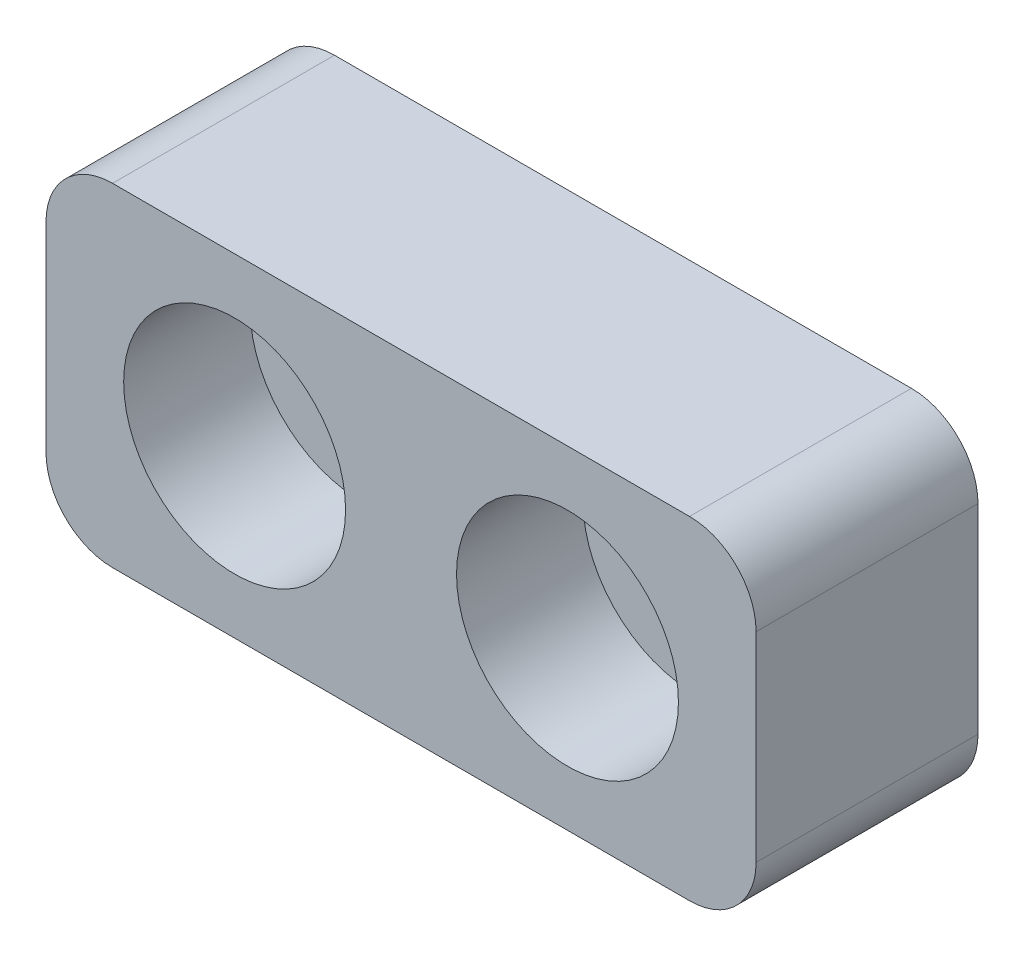
from build123d import *

# Parameters (mm, degrees)
SKETCH1_W                                            = 32
SKETCH1_H                                            = 15
BOSS_EXTRUDE1_DEPTH                                  = 10
CBORE_FOR_M5_HEXAGON_SOCKET_HEAD_CAP_SCR_D           = 5.5
CBORE_FOR_M5_HEXAGON_SOCKET_HEAD_CAP_SCR_DEPTH       = 12.4
CBORE_FOR_M5_HEXAGON_SOCKET_HEAD_CAP_SCR_CBORE_D     = 10
CBORE_FOR_M5_HEXAGON_SOCKET_HEAD_CAP_SCR_CBORE_DEPTH = 5.7
CBORE_FOR_M5_HEXAGON_SOCKET_HEAD_CAP_SCR_TIP         = 1.652366702
FILLET1_R                                            = 3


with BuildPart() as part:
    # Sketch1 → Boss-Extrude1 (new body)
    with BuildSketch(Plane.XY):
        Rectangle(SKETCH1_W, SKETCH1_H)
    extrude(amount=BOSS_EXTRUDE1_DEPTH)

    # CBORE for M5 Hexagon socket head cap screws1
    with Locations(Plane.XY.offset(10)):
        with Locations((7.5, 0), (-7.5, 0)):
            CounterBoreHole(CBORE_FOR_M5_HEXAGON_SOCKET_HEAD_CAP_SCR_D / 2, CBORE_FOR_M5_HEXAGON_SOCKET_HEAD_CAP_SCR_CBORE_D / 2, CBORE_FOR_M5_HEXAGON_SOCKET_HEAD_CAP_SCR_CBORE_DEPTH, depth=CBORE_FOR_M5_HEXAGON_SOCKET_HEAD_CAP_SCR_DEPTH)
            with Locations((0, 0, -(CBORE_FOR_M5_HEXAGON_SOCKET_HEAD_CAP_SCR_DEPTH + CBORE_FOR_M5_HEXAGON_SOCKET_HEAD_CAP_SCR_TIP / 2))):  # 118° drill point
                Cone(0, CBORE_FOR_M5_HEXAGON_SOCKET_HEAD_CAP_SCR_D / 2, CBORE_FOR_M5_HEXAGON_SOCKET_HEAD_CAP_SCR_TIP, mode=Mode.SUBTRACT)

    # Fillet1
    fillet1_edges = [part.edges().sort_by_distance(p)[0] for p in [
        (16, -7.5, 5),
        (-16, -7.5, 5),
        (-16, 7.5, 5),
        (16, 7.5, 5),
    ]]
    fillet(fillet1_edges, radius=FILLET1_R)


solid = part.part
